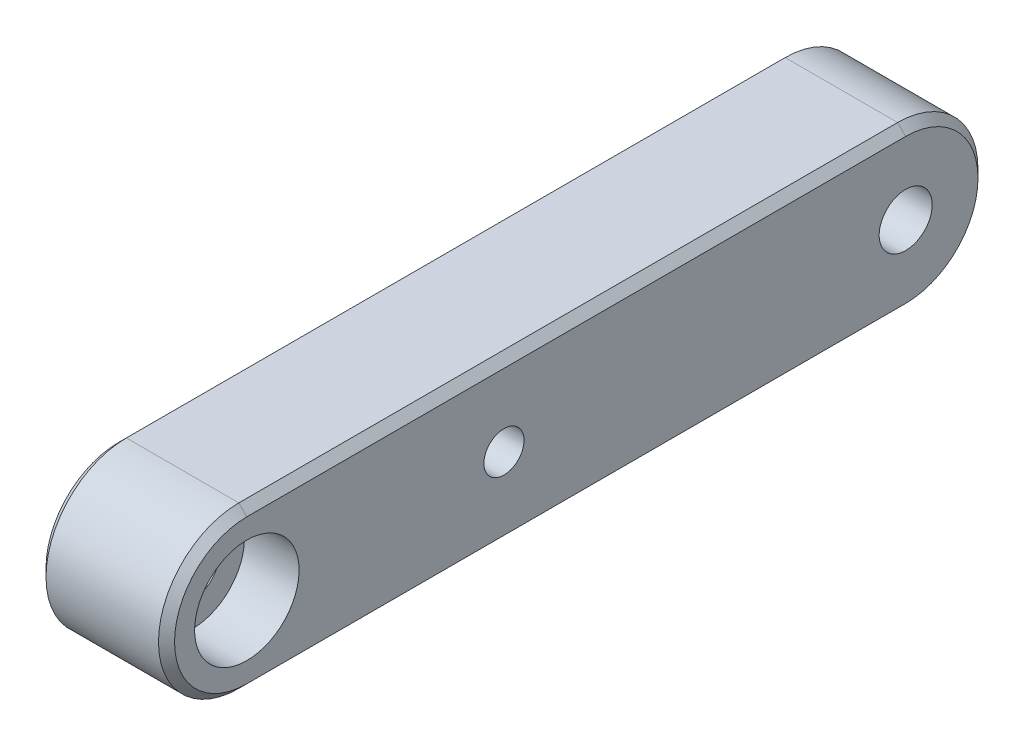
from build123d import *

# Parameters (mm, degrees)
EXTRUDE_1_DEPTH           = 4
HOLE_WIZARD_1_D           = 3.4
HOLE_WIZARD_1_CBORE_D     = 6.5
HOLE_WIZARD_1_CBORE_DEPTH = 3.4
HOLE_WIZARD_M3_1_D        = 2.5
HOLE_WIZARD_M4_1_D        = 3.3
CHAMFER_1_SIZE            = 0.5


with BuildPart() as part:
    # 草图1 → 凸台-拉伸1 (new, symmetric)
    with BuildSketch(Plane(origin=(0, 0, 0), x_dir=(0, 0, -1), z_dir=(1, 0, 0))):
        with BuildLine():
            Line((20.5, -5), (-20.5, -5))
            ThreePointArc((-20.5, -5), (-25.5, 0), (-20.5, 5))
            Line((-20.5, 5), (20.5, 5))
            ThreePointArc((20.5, 5), (25.5, 0), (20.5, -5))
        make_face()
    extrude(amount=EXTRUDE_1_DEPTH, both=True)

    # 打孔尺寸(%根据)内六角圆柱头螺钉的类型1 (through all)
    with Locations(Plane(origin=(4, 0, 0), x_dir=(0, 0, -1), z_dir=(1, 0, 0))):
        with Locations((-20.5, 0)):
            CounterBoreHole(HOLE_WIZARD_1_D / 2, HOLE_WIZARD_1_CBORE_D / 2, HOLE_WIZARD_1_CBORE_DEPTH)

    # M3 螺纹孔1 (through all)
    with Locations(Plane(origin=(4, 0, 0), x_dir=(0, 0, -1), z_dir=(1, 0, 0))):
        with Locations((-4.5, 0)):
            Hole(HOLE_WIZARD_M3_1_D / 2)

    # M4 螺纹孔1 (through all)
    with Locations(Plane(origin=(4, 0, 0), x_dir=(0, 0, -1), z_dir=(1, 0, 0))):
        with Locations((20.5, 0)):
            Hole(HOLE_WIZARD_M4_1_D / 2)

    # 倒角1
    chamfer_1_edges = [part.edges().sort_by_distance(p)[0] for p in [
        (4, 0, 25.5),
        (4, -5, 0),
        (4, 0, -25.5),
        (-4, -5, 0),
        (-4, 0, 25.5),
        (-4, 5, 0),
        (-4, 0, -25.5),
        (4, 5, 0),
    ]]
    chamfer(chamfer_1_edges, length=CHAMFER_1_SIZE)


solid = part.part
